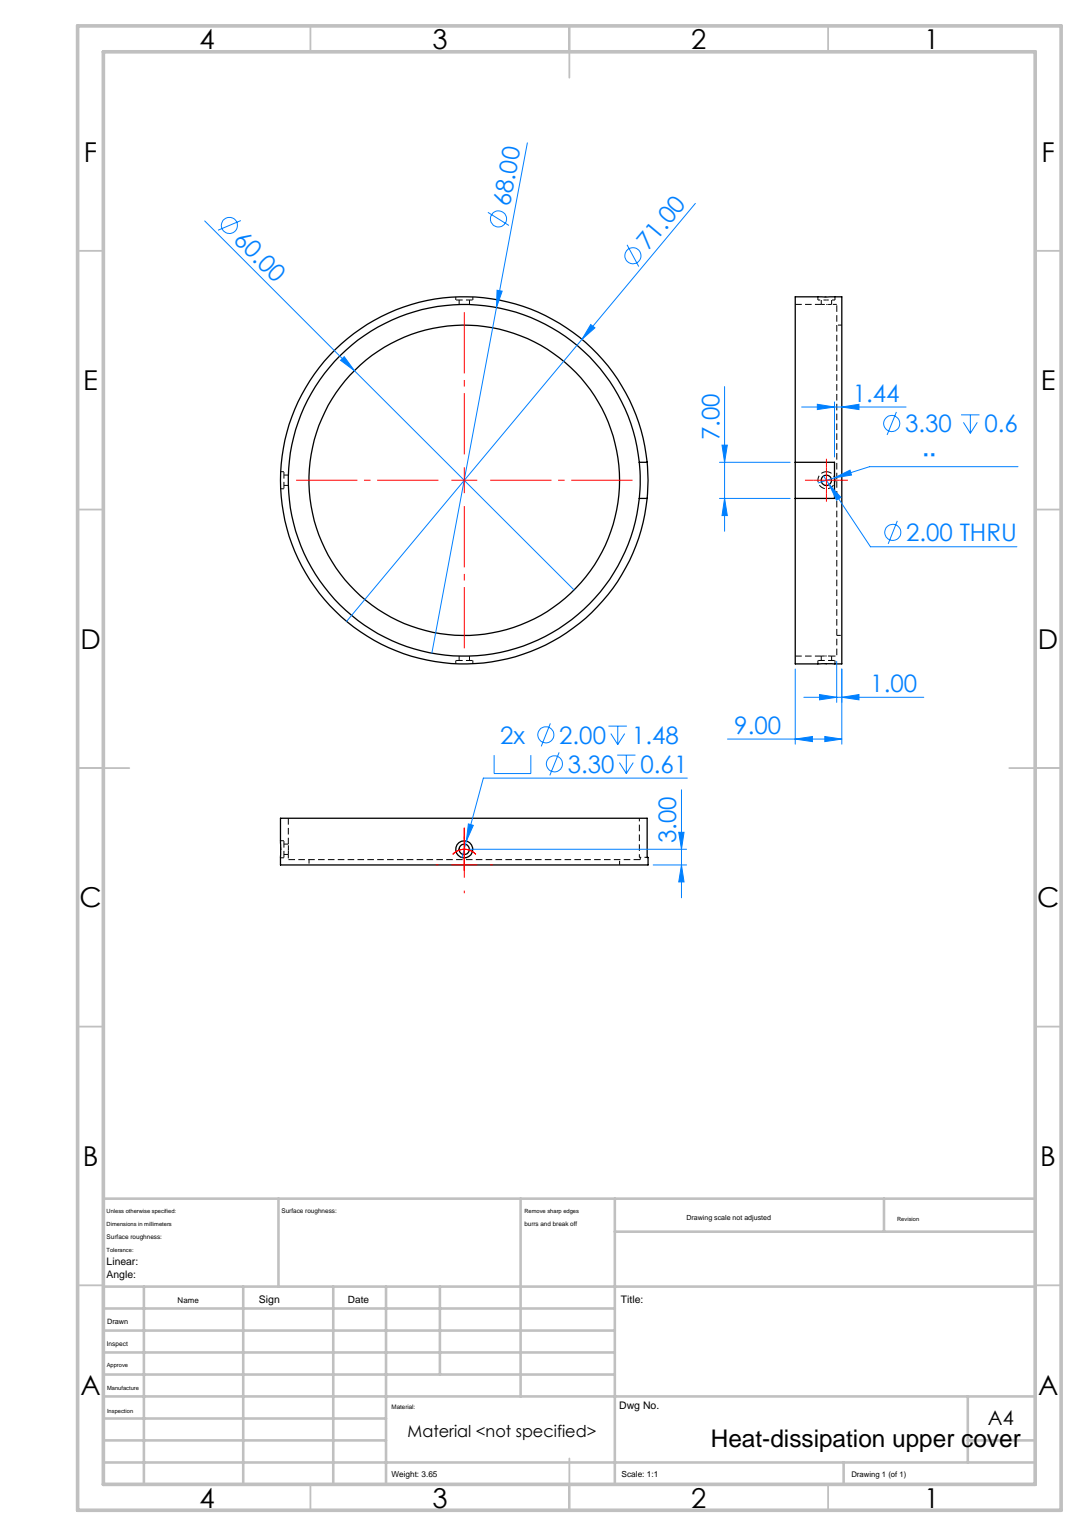
SolidWorks part; units mm, degrees
ref_plane "Front Plane" through (0, 0, 0) normal (0, 0, 1) x (1, 0, 0)
ref_plane "Top Plane" through (0, 0, 0) normal (0, 1, 0) x (1, 0, 0)
ref_plane "Right Plane" through (0, 0, 0) normal (1, 0, 0) x (0, 0, -1)
other "Configuration Table"
sketch "Sketch1" plane through (0, 0, 0) normal (0, 0, 1) x (1, 0, 0)
  line L0 (0, -1.3479) -> (0, 3.3248) construction
  line L1 (-5.2948, 0) -> (6.1657, 0) construction
  line L2 (34, 0) -> (34, 8)
  line L3 (34, 8) -> (30, 8)
  line L4 (30, 8) -> (30, 9)
  line L5 (30, 9) -> (35.5, 9)
  line L6 (35.5, 9) -> (35.5, 0)
  line L7 (35.5, 0) -> (34, 0)
  dimension "D1" = 1
  dimension "D2" = 1.5
  dimension "D3" = 60
  dimension "D4" = 68
  dimension "D5" = 8
revolve "Revolve1" add sketch "Sketch1" angle 360 about L0
sketch "Sketch2" plane through (0, 0, 0) normal (0, 0, 1) x (1, 0, 0)
  line L0 (0, -12.7167) -> (0, 23.8605) construction
  line L2 (-3.5, 7.56) -> (3.5, 7.56)
  line L3 (-3.5, 7.56) -> (-3.5, -2.44)
  line L4 (-3.5, -2.44) -> (3.5, -2.44)
  line L5 (3.5, 7.56) -> (3.5, -2.44)
  line L6 (-3.5, 7.56) -> (3.5, -2.44) construction
  line L7 (-3.5, -2.44) -> (3.5, 7.56) construction
  line L8 (30, 9) -> (-30, 9) construction
  point P3 (0, 2.56)
  dimension "D1" = 1.44
  dimension "D2" = 7
  dimension "D3" = 10
extrude "Cut-Extrude1" cut sketch "Sketch2" against normal through all
sketch "Sketch3" plane through (0, 0, 0) normal (0, 0, 1) x (1, 0, 0)
  line L0 (0, -20.08) -> (0, 27.4393) construction
  line L1 (30, 9) -> (-30, 9) construction
  circle A0 centre (0, 6) radius 1.65
  dimension "D1" = 3.3
  dimension "D2" = 3
extrude "Cut-Extrude2" cut sketch "Sketch3" against normal blind 0.65 and the other way blind 10 from offset 35.5
pattern_circular "CirPattern1" count 4 over 360 about axis through (0, 0, 0) along (0, 1, 0) skipping 2 of "Cut-Extrude2"
sketch "Sketch4" plane through (0, 0, 0) normal (0, 0, 1) x (1, 0, 0)
  line L0 (30, 9) -> (-30, 9) construction
  line L1 (0, 0) -> (0, 20.3046) construction
  circle A0 centre (0, 6) radius 1
  dimension "D1" = 2
  dimension "D2" = 3
extrude "Cut-Extrude3" cut sketch "Sketch4" along normal through all contours A0
pattern_circular "CirPattern3" count 4 over 360 about axis through (0, -1.3479, 0) along (0, -1, 0) skipping 2 of "Cut-Extrude3"
